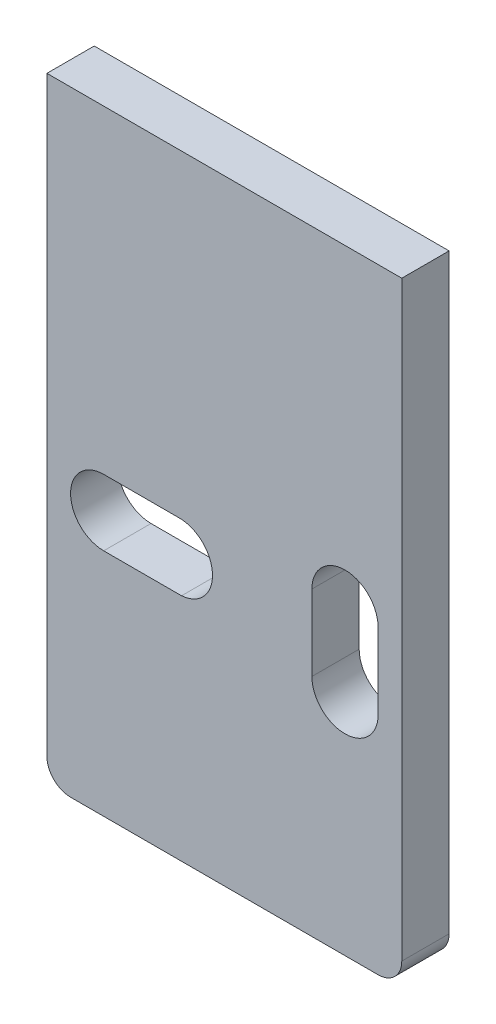
from build123d import *

# Parameters (mm, degrees)
EXTRUDE_1_DEPTH = 10


with BuildPart() as part:
    # 草图1 → 凸台-拉伸1 (new body)
    with BuildSketch(Plane.XY):
        with BuildLine():
            Line((-37.5, 54.4), (-37.5, -70.6))
            ThreePointArc((-37.5, -70.6), (-36.035533906, -74.135533906), (-32.5, -75.6))
            Line((-32.5, -75.6), (32.5, -75.6))
            ThreePointArc((32.5, -75.6), (36.035533906, -74.135533906), (37.5, -70.6))
            Line((37.5, -70.6), (37.5, 54.4))
            Line((37.5, 54.4), (-37.5, 54.4))
        make_face()
        with BuildLine():
            Line((-9.03462289, -27), (-9.029321888, -26.984157939))
            ThreePointArc((-9.029321888, -26.984157939), (-2.503961636, -19.764527679), (-9.5, -13))
            Line((-9.5, -13), (-25.5, -13))
            ThreePointArc((-25.5, -13), (-32.5, -20), (-25.5, -27))
            Line((-25.5, -27), (-9.03462289, -27))
        make_face(mode=Mode.SUBTRACT)
        with BuildLine():
            ThreePointArc((18.5, -28), (25.5, -35), (32.5, -28))
            Line((32.5, -28), (32.5, -12))
            ThreePointArc((32.5, -12), (25.5, -5), (18.5, -12))
            Line((18.5, -12), (18.5, -28))
        make_face(mode=Mode.SUBTRACT)
    extrude(amount=EXTRUDE_1_DEPTH)


solid = part.part
